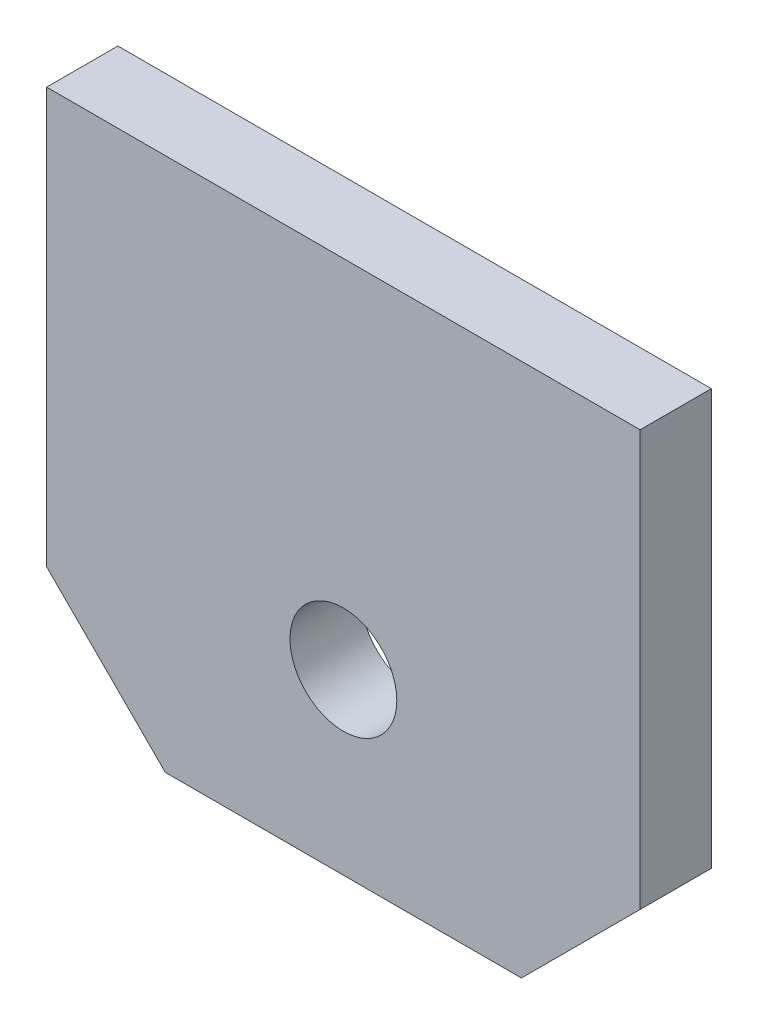
SolidWorks part; units mm, degrees
material "Q235B"
ref_plane "Front" through (0, 0, 0) normal (0, 0, 1) x (1, 0, 0)
ref_plane "Top" through (0, 0, 0) normal (0, 1, 0) x (1, 0, 0)
ref_plane "Right" through (0, 0, 0) normal (1, 0, 0) x (0, 0, -1)
sketch "Sketch1" plane through (0, 0, 0) normal (0, 0, 1) x (1, 0, 0)
  line L1 (-25, -22.5) -> (25, -22.5)
  line L2 (-25, -22.5) -> (-25, 22.5)
  line L3 (-25, 22.5) -> (25, 22.5)
  line L4 (25, -22.5) -> (25, 22.5)
  line L5 (0, 22.5) -> (0, -22.5) construction
  line L6 (-25, 0) -> (25, 0) construction
  point P0 (0, 0)
  dimension "D1" = 50
  dimension "D2" = 45
extrude "Boss-Extrude1" add sketch "Sketch1" along normal blind 6
sketch "Sketch2" plane through (0, 0, 6) normal (0, 0, 1) x (1, 0, 0)
  line L1 (-25, -22.5) -> (25, -22.5) construction
  circle A0 centre (0, -7.5) radius 4.5
  dimension "D1" = 9
  dimension "D2" = 15
extrude "Cut-Extrude1" cut sketch "Sketch2" against normal blind 6
chamfer "Chamfer1" distance 10 angle 45 2 edges at (-25, -22.5, 3) (25, -22.5, 3)
equation "\"零件重量\"= IIF ( \"SW-质量\" > 100 , int ( \"SW-质量\" ) , \"SW-质量\" )"
